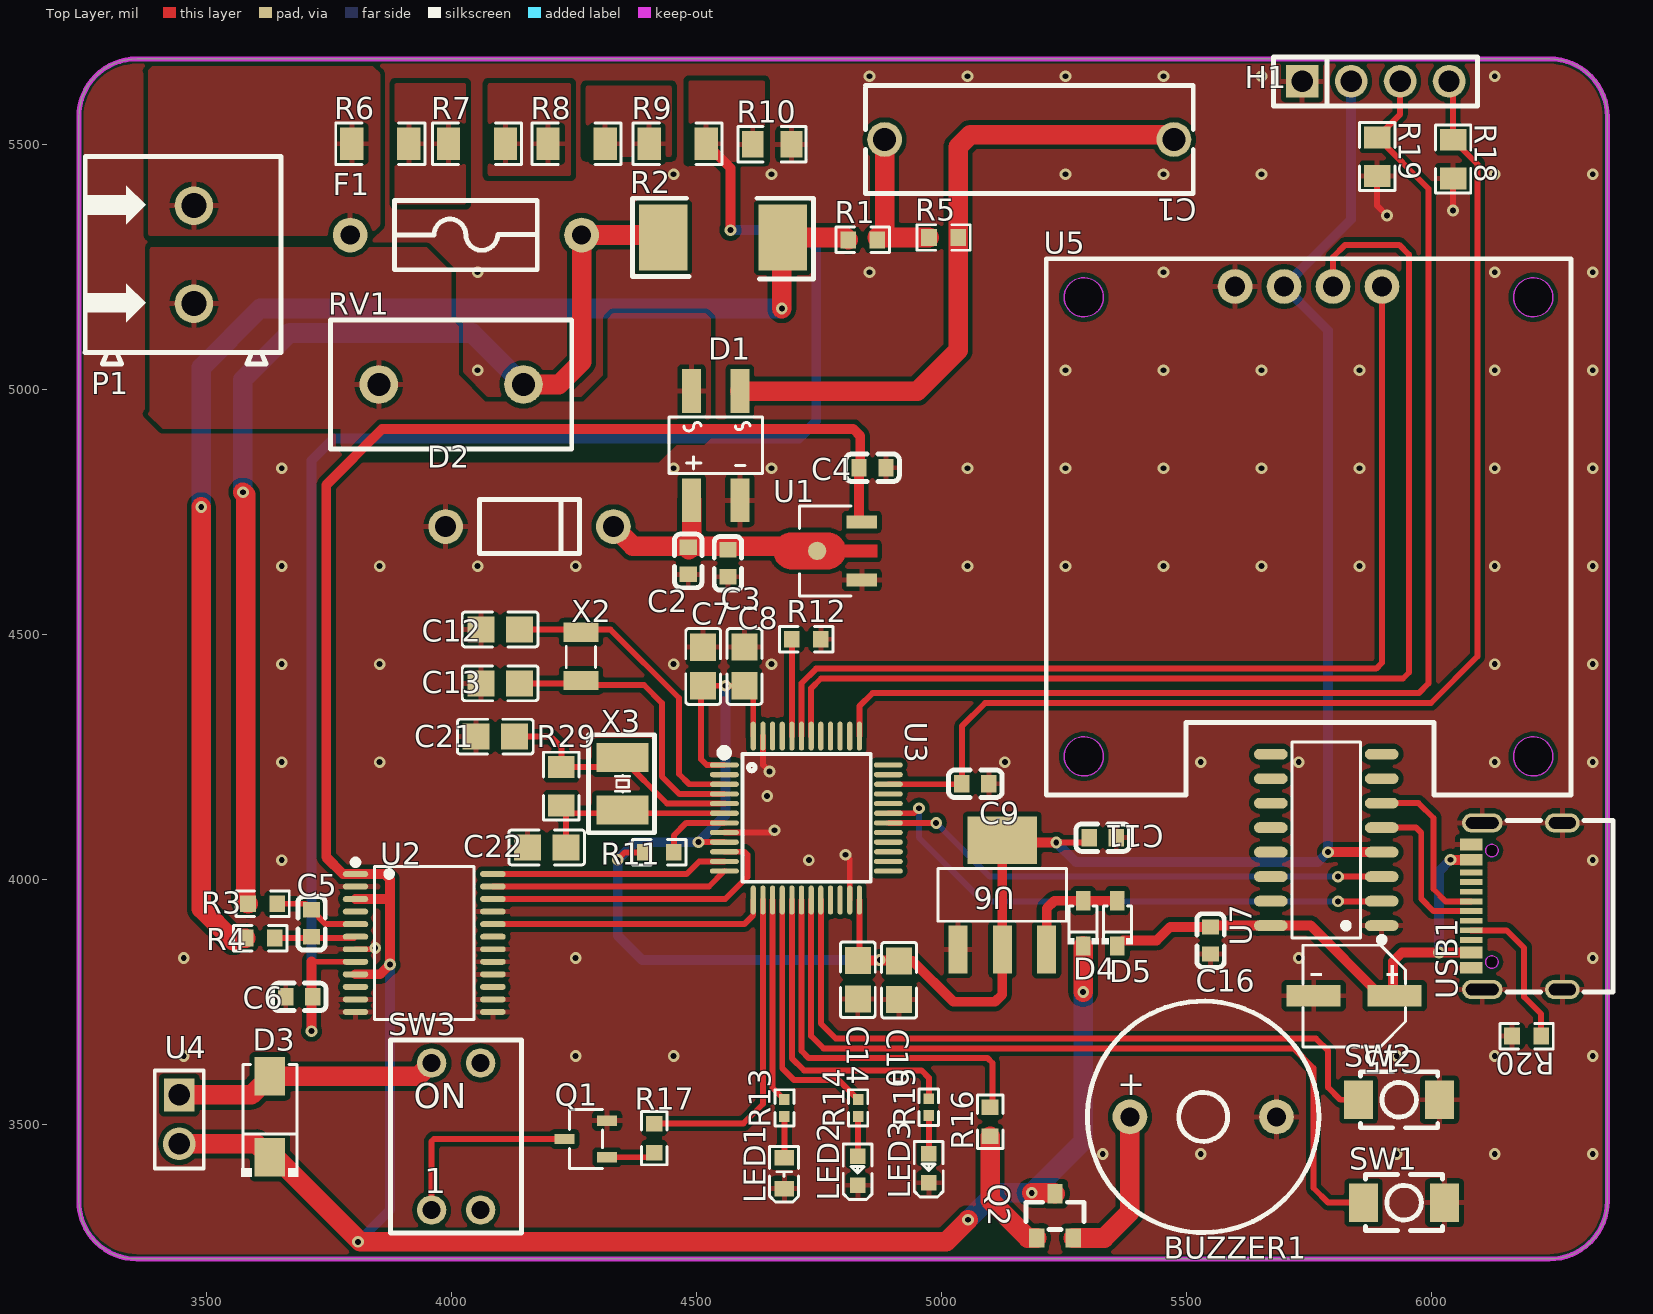
[diagram p0: Top Layer view]
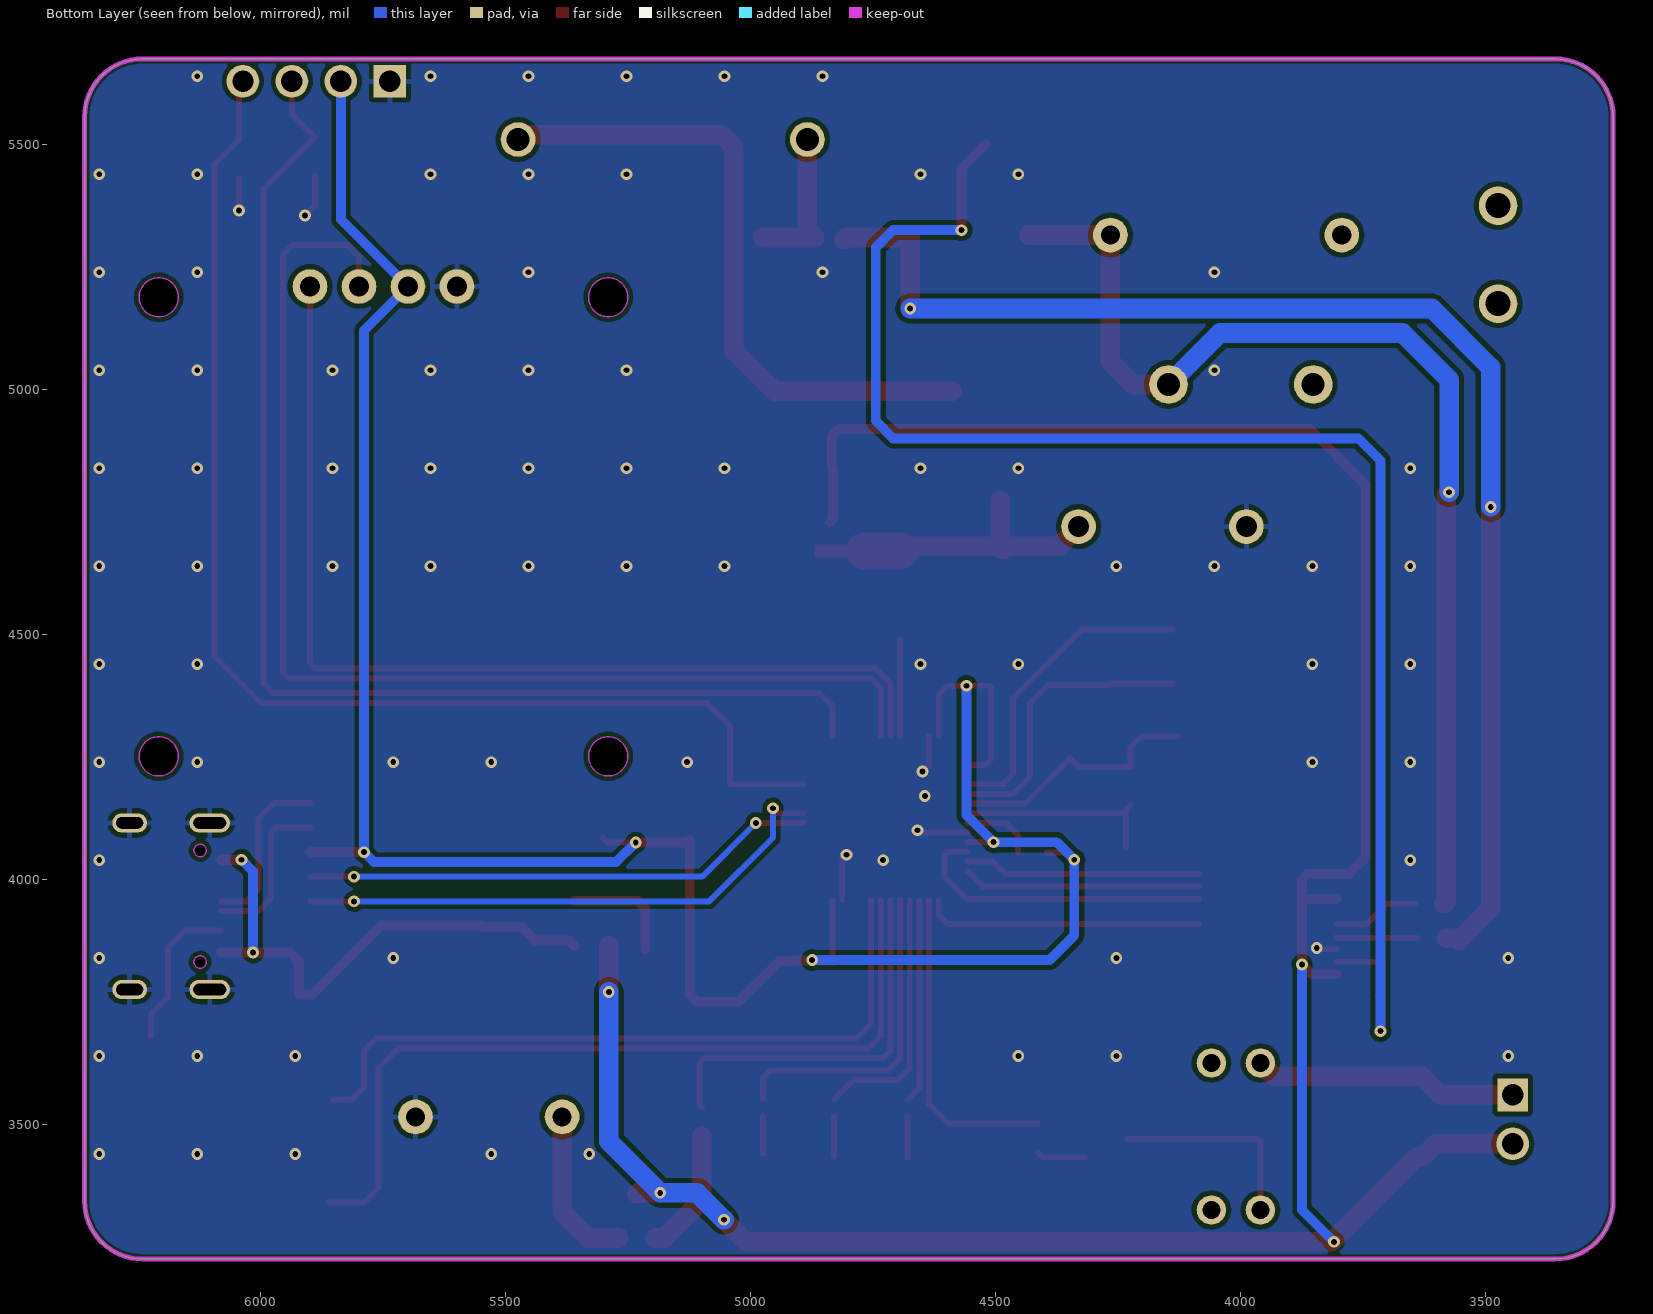
[diagram p1: Bottom Layer view, seen from below]
# Altium PCB MISC61242.pcbdoc
Units mil, origin at the board's own origin, x right, y up, seen from the top; angles counter-clockwise.
Board outline 3120 x 2449.61 mil, 2 copper layers (Top Layer, Bottom Layer), stack 2.757 mil thick; 67 components, 52 nets, 243 pads, 106 vias.

## Layer stack, top to bottom
Top Solder Mask Layer: solder mask 0.394, Dk 3.3
Top Layer: signal copper 1.379
Bottom Layer: signal copper 1.378
Bottom Solder Mask Layer: solder mask 0.394, Dk 3.3

## Board outline
3358.11,5674.61 ccw(c3358.11,5556.5) 3240,5556.5 3240,3343.11 ccw(c3358.11,3343.11) 3358.11,3225 6241.89,3225 ccw(c6241.89,3343.11) 6360,3343.11 6360,5556.5 ccw(c6241.89,5556.5) 6241.89,5674.61 3358.11,5674.61

## Design rules (kind name [scope] priority, off if disabled: settings)
BoardOutlineClearance Plane_innerPlane_1 [All] p2 off: genericclearance=4 ignorepadtopadclearanceinfootprint=FALSE except(0: Arc-SplitContinuation Track-SplitContinuation SMDPad-SplitContinuation THPad-SplitContinuation Via-SplitContinuation Fill-SplitContinuation Region-SplitContinuation Poly-SplitContinuation Text-SplitContinuation Hole-SplitContinuation; 6: Arc-CutoutEdge Track-CutoutEdge SMDPad-CutoutEdge THPad-CutoutEdge Via-CutoutEdge Text-CutoutEdge; 6.9: Hole-OutlineEdge Hole-CutoutEdge; 10: Poly-OutlineEdge Poly-CutoutEdge; 11.8: Arc-OutlineEdge Track-OutlineEdge SMDPad-OutlineEdge THPad-OutlineEdge Via-OutlineEdge Fill-OutlineEdge Region-OutlineEdge Text-OutlineEdge Fill-CutoutEdge Region-CutoutEdge)
BoardOutlineClearance Copper_copperRegion_1 [All] p4 off: genericclearance=4 ignorepadtopadclearanceinfootprint=FALSE except(0: Arc-SplitContinuation Track-SplitContinuation SMDPad-SplitContinuation THPad-SplitContinuation Via-SplitContinuation Fill-SplitContinuation Region-SplitContinuation Poly-SplitContinuation Text-SplitContinuation Hole-SplitContinuation; 6: Arc-CutoutEdge Track-CutoutEdge SMDPad-CutoutEdge THPad-CutoutEdge Via-CutoutEdge Text-CutoutEdge; 6.9: Hole-OutlineEdge Hole-CutoutEdge; 10: Poly-OutlineEdge Poly-CutoutEdge; 11.8: Arc-OutlineEdge Track-OutlineEdge SMDPad-OutlineEdge THPad-OutlineEdge Via-OutlineEdge Fill-OutlineEdge Region-OutlineEdge Text-OutlineEdge Fill-CutoutEdge Region-CutoutEdge)
BoardOutlineClearance Copper_copperRegion_copperThickness1oz_1 [All] p6 off: genericclearance=4 ignorepadtopadclearanceinfootprint=FALSE except(0: Arc-SplitContinuation Track-SplitContinuation SMDPad-SplitContinuation THPad-SplitContinuation Via-SplitContinuation Fill-SplitContinuation Region-SplitContinuation Poly-SplitContinuation Text-SplitContinuation Hole-SplitContinuation; 6: Arc-CutoutEdge Track-CutoutEdge SMDPad-CutoutEdge THPad-CutoutEdge Via-CutoutEdge Text-CutoutEdge; 6.9: Hole-OutlineEdge Hole-CutoutEdge; 10: Poly-OutlineEdge Poly-CutoutEdge; 11.8: Arc-OutlineEdge Track-OutlineEdge SMDPad-OutlineEdge THPad-OutlineEdge Via-OutlineEdge Fill-OutlineEdge Region-OutlineEdge Text-OutlineEdge Fill-CutoutEdge Region-CutoutEdge)
BoardOutlineClearance Copper_copperRegion_Copper_copperRegion_1 [All] p8 off: genericclearance=4 ignorepadtopadclearanceinfootprint=FALSE except(0: Arc-SplitContinuation Track-SplitContinuation SMDPad-SplitContinuation THPad-SplitContinuation Via-SplitContinuation Fill-SplitContinuation Region-SplitContinuation Poly-SplitContinuation Text-SplitContinuation Hole-SplitContinuation; 6: Arc-CutoutEdge Track-CutoutEdge SMDPad-CutoutEdge THPad-CutoutEdge Via-CutoutEdge Text-CutoutEdge; 6.9: Hole-OutlineEdge Hole-CutoutEdge; 10: Poly-OutlineEdge Poly-CutoutEdge; 11.8: Arc-OutlineEdge Track-OutlineEdge SMDPad-OutlineEdge THPad-OutlineEdge Via-OutlineEdge Fill-OutlineEdge Region-OutlineEdge Text-OutlineEdge Fill-CutoutEdge Region-CutoutEdge)
BoardOutlineClearance copperThickness1oz_1 [All] p10: genericclearance=4 ignorepadtopadclearanceinfootprint=FALSE except(0: Arc-SplitContinuation Track-SplitContinuation SMDPad-SplitContinuation THPad-SplitContinuation Via-SplitContinuation Fill-SplitContinuation Region-SplitContinuation Poly-SplitContinuation Text-SplitContinuation Hole-SplitContinuation; 6: Arc-CutoutEdge Track-CutoutEdge SMDPad-CutoutEdge THPad-CutoutEdge Via-CutoutEdge Text-CutoutEdge; 6.9: Hole-OutlineEdge Hole-CutoutEdge; 10: Poly-OutlineEdge Poly-CutoutEdge; 11.8: Arc-OutlineEdge Track-OutlineEdge SMDPad-OutlineEdge THPad-OutlineEdge Via-OutlineEdge Fill-OutlineEdge Region-OutlineEdge Text-OutlineEdge Fill-CutoutEdge Region-CutoutEdge)
Clearance Plane_innerPlane [All] p1 off: gap=4 ignorepadtopadclearanceinfootprint=FALSE except(6: SMDPad-Track SMDPad-SMDPad THPad-Track SMDPad-THPad THPad-THPad Track-Via SMDPad-Via THPad-Via Via-Via Fill-SMDPad Region-SMDPad Fill-THPad Region-THPad Fill-Via Region-Via Fill-Fill Fill-Region Region-Region Arc-Track Arc-SMDPad Arc-THPad Arc-Via Fill-Arc Region-Arc Arc-Arc Text-Track SMDPad-Text Text-THPad Text-Via Fill-Text Region-Text Arc-Text Text-Text; 6.9: Hole-Track Hole-SMDPad Hole-THPad Hole-Via Fill-Hole Region-Hole Hole-Arc Hole-Text; 10: Poly-Track Poly-SMDPad Poly-THPad Poly-Via Poly-Fill Poly-Region Poly-Poly Poly-Arc Poly-Text Poly-Hole; 11.8: Fill-Track Region-Track)
Clearance Copper_copperRegion [All] p3 off: gap=4 ignorepadtopadclearanceinfootprint=FALSE except(6: SMDPad-Track SMDPad-SMDPad THPad-Track SMDPad-THPad THPad-THPad Track-Via SMDPad-Via THPad-Via Via-Via Fill-SMDPad Region-SMDPad Fill-THPad Region-THPad Fill-Via Region-Via Fill-Fill Fill-Region Region-Region Arc-Track Arc-SMDPad Arc-THPad Arc-Via Fill-Arc Region-Arc Arc-Arc Text-Track SMDPad-Text Text-THPad Text-Via Fill-Text Region-Text Arc-Text Text-Text; 6.9: Hole-Track Hole-SMDPad Hole-THPad Hole-Via Fill-Hole Region-Hole Hole-Arc Hole-Text; 10: Poly-Track Poly-SMDPad Poly-THPad Poly-Via Poly-Fill Poly-Region Poly-Poly Poly-Arc Poly-Text Poly-Hole; 11.8: Fill-Track Region-Track)
Clearance Copper_copperRegion_copperThickness1oz [All] p5 off: gap=4 ignorepadtopadclearanceinfootprint=FALSE except(6: SMDPad-Track SMDPad-SMDPad THPad-Track SMDPad-THPad THPad-THPad Track-Via SMDPad-Via THPad-Via Via-Via Fill-SMDPad Region-SMDPad Fill-THPad Region-THPad Fill-Via Region-Via Fill-Fill Fill-Region Region-Region Arc-Track Arc-SMDPad Arc-THPad Arc-Via Fill-Arc Region-Arc Arc-Arc Text-Track SMDPad-Text Text-THPad Text-Via Fill-Text Region-Text Arc-Text Text-Text; 6.9: Hole-Track Hole-SMDPad Hole-THPad Hole-Via Fill-Hole Region-Hole Hole-Arc Hole-Text; 10: Poly-Track Poly-SMDPad Poly-THPad Poly-Via Poly-Fill Poly-Region Poly-Poly Poly-Arc Poly-Text Poly-Hole; 11.8: Fill-Track Region-Track)
Clearance Copper_copperRegion_Copper_copperRegion [All] p7 off: gap=4 ignorepadtopadclearanceinfootprint=FALSE except(6: SMDPad-Track SMDPad-SMDPad THPad-Track SMDPad-THPad THPad-THPad Track-Via SMDPad-Via THPad-Via Via-Via Fill-SMDPad Region-SMDPad Fill-THPad Region-THPad Fill-Via Region-Via Fill-Fill Fill-Region Region-Region Arc-Track Arc-SMDPad Arc-THPad Arc-Via Fill-Arc Region-Arc Arc-Arc Text-Track SMDPad-Text Text-THPad Text-Via Fill-Text Region-Text Arc-Text Text-Text; 6.9: Hole-Track Hole-SMDPad Hole-THPad Hole-Via Fill-Hole Region-Hole Hole-Arc Hole-Text; 10: Poly-Track Poly-SMDPad Poly-THPad Poly-Via Poly-Fill Poly-Region Poly-Poly Poly-Arc Poly-Text Poly-Hole; 11.8: Fill-Track Region-Track)
Clearance copperThickness1oz [All] p9: gap=4 ignorepadtopadclearanceinfootprint=FALSE except(6: SMDPad-Track SMDPad-SMDPad THPad-Track SMDPad-THPad THPad-THPad Track-Via SMDPad-Via THPad-Via Via-Via Fill-SMDPad Region-SMDPad Fill-THPad Region-THPad Fill-Via Region-Via Fill-Fill Fill-Region Region-Region Arc-Track Arc-SMDPad Arc-THPad Arc-Via Fill-Arc Region-Arc Arc-Arc Text-Track SMDPad-Text Text-THPad Text-Via Fill-Text Region-Text Arc-Text Text-Text; 6.9: Hole-Track Hole-SMDPad Hole-THPad Hole-Via Fill-Hole Region-Hole Hole-Arc Hole-Text; 10: Poly-Track Poly-SMDPad Poly-THPad Poly-Via Poly-Fill Poly-Region Poly-Poly Poly-Arc Poly-Text Poly-Hole; 11.8: Fill-Track Region-Track)
DiffPairsRouting differentialPair [All] p1: maxlimit=6 minlimit=5 mostfreqgap=6 toplayer_minwidth=5 toplayer_prefwidth=100 toplayer_maxwidth=100 toplayer_mingap=5 toplayer_prefgap=6 toplayer_maxgap=6 bottomlayer_minwidth=5 bottomlayer_prefwidth=100 bottomlayer_maxwidth=100 bottomlayer_mingap=5 bottomlayer_prefgap=6 bottomlayer_maxgap=6 maxuncoupledlength=10
HoleToHoleClearance otherClearance [All] p1: gap=11.8 allowstackedmicrovias=TRUE
Length netLength [All] p1: minlimit=0 maxlimit=0
PasteMaskExpansion pasteMaskExpansion [All] p1: expansion=0
PlaneConnect innerPlane [All] p1: planeconnectstyle=Relief reliefexpansion=20 reliefentries=4 reliefconductorwidth=10 reliefairgap=10
PolygonConnect copperRegion_copperThickness1oz [All] p1 off: connectstyle=Relief reliefconductorwidth=10 reliefentries=4 polygonreliefangle="90 Angle" airgapwidth=10 via.connectstyle=Relief via.reliefconductorwidth=10 via.reliefentries=4 via.polygonreliefangle="90 Angle" via.airgapwidth=10
PolygonConnect copperRegion_Copper_copperRegion [All] p2 off: connectstyle=Relief reliefconductorwidth=10 reliefentries=4 polygonreliefangle="90 Angle" airgapwidth=10 via.connectstyle=Relief via.reliefconductorwidth=10 via.reliefentries=4 via.polygonreliefangle="90 Angle" via.airgapwidth=10
PolygonConnect copperRegion [All] p3: connectstyle=Direct reliefconductorwidth=10 reliefentries=4 polygonreliefangle="90 Angle" airgapwidth=10 via.connectstyle=Relief via.reliefconductorwidth=10 via.reliefentries=4 via.polygonreliefangle="90 Angle" via.airgapwidth=10
RoutingVias viaSize [All] p1: holewidth=12 width=24 viastyle="Through Hole" minholewidth=1 minwidth=1 maxholewidth=393.7 maxwidth=248
SolderMaskExpansion solderMaskExpansion [IsVia] p1: expansion=-1000 istentingtop=TRUE
SolderMaskExpansion solderMaskExpansion [All] p2: expansion=2 istentingtop=FALSE
Width copperThickness1oz_2 [All] p1: maxlimit=100 minlimit=5 preferedwidth=10

## Components (designator, comment, footprint, x,y, rotation, side; value= is the part's Value field where it differs from the comment)
BUZZER1 "2.4kHz" BUZ-TH_BD12.0-P7.60-D0.6-FD 5535,3515 r0 top
C1 "470nF" CAP-TH_L17.0-W5.5-P15.00-D1.2 5180,5510 r180 top
C2 "47uF" C0603 4484.01,4649.76 r270 top
C3 "0.1μF" C0603 4565,4645 r270 top
C4 "10μF" C0603 4860,4840 r180 top
C5 "1nF" C0603 3715,3910 r90 top
C6 "1nF" C0603 3690,3760 r0 top
C7 "100nF" C0805 4514.37,4434.37 r90 top
C8 "100nF" C0805 4598.8,4434.51 r270 top
C9 "100nF" C0603 5070,4195 r180 top
C10 "100nF" C0805 4914.37,3793.97 r270 top
C11 "100nF" C0603 5330,4085 r180 top
C12 "20pF" C0805 4100,4510 r180 top
C13 "20pF" C0805 4100,4400 r0 top
C14 "100nF" C0805 4830,3795 r90 top
C15 "10uF" CAP-SMD_BD5.0-L5.3-W5.3-FD 5843.3,3762.26 r180 top
C16 "100nF" C0603 5550,3875 r90 top
C21 "20pF" C0805 4090.21,4291.12 r0 top
C22 "20pF" C0805 4195,4065 r0 top
D1 "MB10S" MBS_L4.7-W4.0-P2.50-LS7.0-TL 4540,4885 r270 top
D2 "1N4742" DO-41_BD2.4-L4.7-P8.70-D0.8-FD 4160,4720 r0 top
D3 "1N4007" SMA_L4.3-W2.5-LS5.0-RD 3630,3515 r90 top
D4 "1N5819WS" SOD-323_L1.8-W1.3-LS2.5-RD 5290,3910 r90 top
D5 "1N5819WS" SOD-323_L1.8-W1.3-LS2.5-RD 5360,3910 r90 top
F1 "2F.0500212000S1B02" FUSE-TH_BD3.0-L7.2-P11.20-D0.6 4030,5315 r0 top
H1 "" HDR-TH_4P-P2.54-V-F 5887,5628.78 r0 top
LED1 "NCD0603G1" LED0603-RD_1 4679.87,3400.05 r90 top
LED2 "NCD0603R1" LED0603-RD_RED 4830,3405 r90 top
LED3 "NCD0603Y1" LED0603-RD 4975,3410 r90 top
P1 "WJ500V-5.08-2P" CONN-TH_2P-P5.00_WJ500V-5.08-2P 3475,5275 r90 top
Q1 "S8050 J3Y(RANGE:200-350)" SOT-23-3_L3.0-W1.7-P0.95-LS2.9-BR 4275,3470 r0 top
Q2 "" S8050_SOT-23 5232.54,3313.14 r270 top
R1 "10Ω" R0603 4840,5305 r0 top
R2 "2mΩ" RES-SMD_L6.4-W3.2-1 4555,5310 r0 top
R3 "1K" R0603 3615,3950 r0 top
R4 "1K" R0603 3610,3880 r0 top
R5 "1MΩ" R0603 5005,5310 r0 top
R6 "1MΩ" R1206 3855.45,5501.36 r0 top
R7 "1MΩ" R1206 4052.86,5501.36 r0 top
R8 "1MΩ" R1206 4256.06,5501.36 r0 top
R9 "1MΩ" R1206 4462.27,5501.36 r0 top
R10 "10kΩ" R0805 4655,5500 r0 top
R11 "10K" R0603 4425,4055 r0 top
R12 "10K" R0603 4725,4490 r0 top
R13 "220Ω" R0402 4680.3,3533.26 r90 top
R14 "220Ω" R0402 4830.69,3533.26 r90 top
R15 "220Ω" R0402 4975,3535 r90 top
R16 "1KΩ" R0603 5100,3505 r90 top
R17 "1KΩ" R0603 4414.48,3471.81 r270 top
R18 "10kΩ" R0805 6045,5470 r270 top
R19 "10kΩ" R0805 5890,5475 r270 top
R20 "5.1K" R0603 6195,3680 r180 top
R29 "1M" R0805 4225,4190 r90 top
RV1 "190pF@1kHz" RES-TH_L12.5-W6.7-P7.50-D1.2 4000,5010 r0 top
SW1 "TS3425A2P 250gf" SW-SMD_L3.9-W2.9-LS5.0 5945,3340 r0 top
SW2 "TS3425A2P 250gf" SW-SMD_L3.9-W2.9-LS5.0 5935,3550 r0 top
SW3 "BSE02GR" SW-TH_4P-L9.9-W6.8-P7.62-BL 4010,3475 r0 top
U1 "HT7550-1" SOT-89_L4.5-W2.5-P1.50-LS4.2-BR 4785,4670 r0 top
U2 "ADE7755ARSZ" SSOP-24_L8.1-W5.3-P0.65-LS7.8-BL 3945,3870 r270 top
U3 "STM32F030C8T6TR" LQFP-48_L7.0-W7.0-P0.50-LS9.0-BL 4725,4125 r270 top
U4 "KF301-5.0-2P" HDR-M-2.54_1X2 3445,3510 r270 top
U5 "HS96L03W2C03" OLED-TH_L27.8-W27.2-P2.54_C9900033791 5750,5210 r0 top
U6 "AMS1117-3.3" SOT-223-4_L6.5-W3.5-P2.30-LS7.0-BR 5125,3968.34 r270 top
U7 "CH340C" SOP-16_L10.0-W3.9-P1.27-LS6.0-BL 5786.23,4080.41 r90 top
USB1 "TYPE-C16PIN" USB-C-SMD_TYPE-C16PIN 6175,3945 r90 top
X2 "32.768kHz" CRYSTAL-SMD_L3.2-W1.5-FC-135R32.7680KF-A3 4265,4455 r270 top
X3 "8MHz" CRYSTAL-SMD_L3.2-W2.5_3225-8MHZ 4350,4195 r90 top

## Footprints (in the part's own frame and the unit in brackets; to place one, negate y for a bottom-side part, rotate by r counter-clockwise, add the part's x,y. Pads: shape width x height; smd on the part's side, far side on the other; paste and mask are expansions set on the pad)
BUZ-TH_BD12.0-P7.60-D0.6-FD [mm]
  round 1.8 hole 1: 1(-3.8,0) 2(3.8,0)
  silkscreen extent -6,-6 6,6
C0603 [mm]
  rect 0.8x0.9 smd: 1(-0.7,0) 2(0.7,0)
  silkscreen extent -1.39,-0.71 1.39,0.71
C0805 [mm]
  rect 1.41x1.35 smd paste-100 mask+0.051: 1(-1,0) 2(1,0)
  silkscreen extent -1.96,-0.9 1.96,0.9
CAP-SMD_BD5.0-L5.3-W5.3-FD [mm]
  rect 2.8x1.1 smd: 1(-2.1,0) 2(2.1,0)
  silkscreen extent -2.66,-2.62 2.66,2.65
CAP-TH_L17.0-W5.5-P15.00-D1.2 [mm]
  round 1.8 hole 1.2: 1(-7.501,0) 2(7.501,0)
  silkscreen extent -8.5,-2.8 8.5,2.8
CONN-TH_2P-P5.00_WJ500V-5.08-2P [mm]
  round 2 hole 1.3: 1(-2.54,0) 2(2.54,0)
  silkscreen extent -5.68,-4.52 5.08,5.64
CRYSTAL-SMD_L3.2-W1.5-FC-135R32.7680KF-A3 [mm]
  rect 1x1.8 smd paste+0 mask+0.05: 1(-1.25,0) 2(1.25,0)
  silkscreen extent -0.51,-0.76 0.57,0.76
CRYSTAL-SMD_L3.2-W2.5_3225-8MHZ [mil]
  rect 60x106.3 smd paste+0 mask+1.97: 1(-53.62,0) 2(53.62,0)
  silkscreen extent -100,-65 100,70
DO-41_BD2.4-L4.7-P8.70-D0.8-FD [mm]
  round 1.8 hole 1.1: 1(-4.35,0) 2(4.35,0)
  silkscreen extent -2.6,-1.4 2.6,1.4
FUSE-TH_BD3.0-L7.2-P11.20-D0.6 [mm]
  round 1.8 hole 1: 1(-6,0) 2(6,0)
  silkscreen extent -3.7,-1.8 3.7,1.8
HDR-M-2.54_1X2 [mm]
  rect 1.7x1.575 hole 1.1: 1(-1.27,0)
  round 1.7 hole 1.1: 2(1.27,0)
  silkscreen extent -2.54,-1.27 2.54,1.27
HDR-TH_4P-P2.54-V-F [mm]
  rect 1.7x1.7 hole 1.1: 1(-3.81,0)
  round 1.7 hole 1.1: 2(-1.27,0) 3(1.27,0) 4(3.81,0)
  silkscreen extent -5.29,-1.27 5.29,1.27
LED0603-RD [mm]
  rect 0.8x0.8 smd: 1(-0.749,0) 2(0.749,0)
  silkscreen extent -1.49,-0.75 1.39,0.76
LED0603-RD_1 [mm]
  rect 0.8x1 smd: 1(-0.799,-0.004) 2(0.799,0.004)
  silkscreen extent -1.49,-0.75 1.39,0.76
LED0603-RD_RED [mm]
  rect 0.8x0.8 smd: 1(-0.749,-0.003) 2(0.749,0.003)
  silkscreen extent -1.49,-0.75 1.39,0.76
LQFP-48_L7.0-W7.0-P0.50-LS9.0-BL [mm]
  oval 0.27x1.5 smd paste+0 mask+0.05: 1(-2.75,-4.25) 2(-2.25,-4.25) 3(-1.75,-4.25) 4(-1.25,-4.25) 5(-0.75,-4.25) 6(-0.25,-4.25) 7(0.25,-4.25) 8(0.75,-4.25) 9(1.25,-4.25) 10(1.75,-4.25) 11(2.25,-4.25) 12(2.75,-4.25) 25(2.75,4.25) 26(2.25,4.25) 27(1.75,4.25) 28(1.25,4.25) 29(0.75,4.25) 30(0.25,4.25) 31(-0.25,4.25) 32(-0.75,4.25) 33(-1.25,4.25) 34(-1.75,4.25) 35(-2.25,4.25) 36(-2.75,4.25)
  oval 1.5x0.27 smd paste+0 mask+0.05: 13(4.25,-2.75) 14(4.25,-2.25) 15(4.25,-1.75) 16(4.25,-1.25) 17(4.25,-0.75) 18(4.25,-0.25) 19(4.25,0.25) 20(4.25,0.75) 21(4.25,1.25) 22(4.25,1.75) 23(4.25,2.25) 24(4.25,2.75) 37(-4.25,2.75) 38(-4.25,2.25) 39(-4.25,1.75) 40(-4.25,1.25) 41(-4.25,0.75) 42(-4.25,0.25) 43(-4.25,-0.25) 44(-4.25,-0.75) 45(-4.25,-1.25) 46(-4.25,-1.75) 47(-4.25,-2.25) 48(-4.25,-2.75)
  silkscreen extent -3.59,-4.46 3.3,3.34
MBS_L4.7-W4.0-P2.50-LS7.0-TL [mm]
  rect 2.265x0.98 smd: 1(-2.832,1.25) 2(-2.832,-1.25) 3(2.832,-1.25) 4(2.832,1.25)
  silkscreen extent -1.5,-2.43 1.44,2.43
OLED-TH_L27.8-W27.2-P2.54_C9900033791 [mm]
  round 1.8 hole 1.05 paste+0 mask+0.05: 1(-3.81,0) 2(-1.27,0) 3(1.27,0) 4(3.81,0)
  Board Outline Layer circle w0.003: c-11.65,-0.56 r1.016
  Board Outline Layer circle w0.003: c11.65,-0.56 r1.016
  Board Outline Layer circle w0.003: c-11.65,-24.36 r1.016
  Board Outline Layer circle w0.003: c11.65,-24.36 r1.016
  Board Outline Layer region: -10.634,-0.56 -10.735,-1.001 -11.016,-1.354 -11.424,-1.551 -11.876,-1.551 -12.283,-1.354 -12.565,-1.001 -12.666,-0.56 -12.666,-0.56 -12.565,-0.119 -12.283,0.234 -11.876,0.431 -11.424,0.431 -11.016,0.234 -10.735,-0.119 -10.634,-0.56
  Board Outline Layer region: -10.634,-0.56 -10.643,-0.698 -10.672,-0.834 -10.718,-0.965 -10.782,-1.088 -10.862,-1.201 -10.956,-1.303 -11.064,-1.39 -11.183,-1.462 -11.31,-1.517 -11.443,-1.555 -11.581,-1.574 -11.719,-1.574 -11.857,-1.555 -11.99,-1.517 -12.117,-1.462 -12.236,-1.39 -12.343,-1.303 -12.438,-1.201 -12.518,-1.088 -12.582,-0.965 -12.628,-0.834 -12.656,-0.698 -12.666,-0.56 -12.656,-0.422 -12.628,-0.286 -12.582,-0.155 -12.518,-0.032 -12.438,0.081 -12.343,0.183 -12.236,0.27 -12.117,0.342 -11.99,0.397 -11.857,0.435 -11.719,0.454 -11.581,0.454 -11.443,0.435 -11.31,0.397 -11.183,0.342 -11.064,0.27 -10.956,0.183 -10.862,0.081 -10.782,-0.032 -10.718,-0.155 -10.672,-0.286 -10.643,-0.422
  Board Outline Layer region: 12.666,-0.56 12.565,-1.001 12.283,-1.354 11.876,-1.551 11.424,-1.551 11.017,-1.354 10.735,-1.001 10.634,-0.56 10.634,-0.56 10.735,-0.119 11.017,0.234 11.424,0.431 11.876,0.431 12.283,0.234 12.565,-0.119 12.666,-0.56
  Board Outline Layer region: 12.666,-0.56 12.657,-0.698 12.628,-0.834 12.582,-0.965 12.518,-1.088 12.438,-1.201 12.343,-1.303 12.236,-1.39 12.117,-1.462 11.99,-1.517 11.857,-1.555 11.719,-1.574 11.581,-1.574 11.443,-1.555 11.31,-1.517 11.183,-1.462 11.064,-1.39 10.957,-1.303 10.862,-1.201 10.782,-1.088 10.718,-0.965 10.672,-0.834 10.643,-0.698 10.634,-0.56 10.643,-0.422 10.672,-0.286 10.718,-0.155 10.782,-0.032 10.862,0.081 10.957,0.183 11.064,0.27 11.183,0.342 11.31,0.397 11.443,0.435 11.581,0.454 11.719,0.454 11.857,0.435 11.99,0.397 12.117,0.342 12.236,0.27 12.343,0.183 12.438,0.081 12.518,-0.032 12.582,-0.155 12.628,-0.286 12.657,-0.422
  Board Outline Layer region: -10.634,-24.36 -10.735,-24.801 -11.016,-25.154 -11.424,-25.35 -11.876,-25.35 -12.283,-25.154 -12.565,-24.801 -12.666,-24.36 -12.666,-24.36 -12.565,-23.919 -12.283,-23.566 -11.876,-23.369 -11.424,-23.369 -11.016,-23.566 -10.735,-23.919 -10.634,-24.36
  Board Outline Layer region: -10.634,-24.36 -10.643,-24.498 -10.672,-24.634 -10.718,-24.765 -10.782,-24.888 -10.862,-25.001 -10.956,-25.102 -11.064,-25.19 -11.183,-25.262 -11.31,-25.317 -11.443,-25.355 -11.581,-25.374 -11.719,-25.374 -11.857,-25.355 -11.99,-25.317 -12.117,-25.262 -12.236,-25.19 -12.343,-25.102 -12.438,-25.001 -12.518,-24.888 -12.582,-24.765 -12.628,-24.634 -12.656,-24.498 -12.666,-24.36 -12.656,-24.222 -12.628,-24.086 -12.582,-23.955 -12.518,-23.832 -12.438,-23.719 -12.343,-23.617 -12.236,-23.53 -12.117,-23.458 -11.99,-23.403 -11.857,-23.365 -11.719,-23.346 -11.581,-23.346 -11.443,-23.365 -11.31,-23.403 -11.183,-23.458 -11.064,-23.53 -10.956,-23.617 -10.862,-23.719 -10.782,-23.832 -10.718,-23.955 -10.672,-24.086 -10.643,-24.222
  Board Outline Layer region: 12.666,-24.36 12.565,-24.801 12.283,-25.154 11.876,-25.35 11.424,-25.35 11.017,-25.154 10.735,-24.801 10.634,-24.36 10.634,-24.36 10.735,-23.919 11.017,-23.566 11.424,-23.369 11.876,-23.369 12.283,-23.566 12.565,-23.919 12.666,-24.36
  Board Outline Layer region: 12.666,-24.36 12.657,-24.498 12.628,-24.634 12.582,-24.765 12.518,-24.888 12.438,-25.001 12.343,-25.102 12.236,-25.19 12.117,-25.262 11.99,-25.317 11.857,-25.355 11.719,-25.374 11.581,-25.374 11.443,-25.355 11.31,-25.317 11.183,-25.262 11.064,-25.19 10.957,-25.102 10.862,-25.001 10.782,-24.888 10.718,-24.765 10.672,-24.634 10.643,-24.498 10.634,-24.36 10.643,-24.222 10.672,-24.086 10.718,-23.955 10.782,-23.832 10.862,-23.719 10.957,-23.617 11.064,-23.53 11.183,-23.458 11.31,-23.403 11.443,-23.365 11.581,-23.346 11.719,-23.346 11.857,-23.365 11.99,-23.403 12.117,-23.458 12.236,-23.53 12.343,-23.617 12.438,-23.719 12.518,-23.832 12.582,-23.955 12.628,-24.086 12.657,-24.222
  Multi-Layer board cut-out: -10.634,-0.56 -10.735,-1.001 -11.016,-1.354 -11.424,-1.551 -11.876,-1.551 -12.283,-1.354 -12.565,-1.001 -12.666,-0.56 -12.666,-0.56 -12.565,-0.119 -12.283,0.234 -11.876,0.431 -11.424,0.431 -11.016,0.234 -10.735,-0.119 -10.634,-0.56
  Multi-Layer board cut-out: 12.666,-0.56 12.565,-1.001 12.283,-1.354 11.876,-1.551 11.424,-1.551 11.017,-1.354 10.735,-1.001 10.634,-0.56 10.634,-0.56 10.735,-0.119 11.017,0.234 11.424,0.431 11.876,0.431 12.283,0.234 12.565,-0.119 12.666,-0.56
  Multi-Layer board cut-out: -10.634,-24.36 -10.735,-24.801 -11.016,-25.154 -11.424,-25.35 -11.876,-25.35 -12.283,-25.154 -12.565,-24.801 -12.666,-24.36 -12.666,-24.36 -12.565,-23.919 -12.283,-23.566 -11.876,-23.369 -11.424,-23.369 -11.016,-23.566 -10.735,-23.919 -10.634,-24.36
  Multi-Layer board cut-out: 12.666,-24.36 12.565,-24.801 12.283,-25.154 11.876,-25.35 11.424,-25.35 11.017,-25.154 10.735,-24.801 10.634,-24.36 10.634,-24.36 10.735,-23.919 11.017,-23.566 11.424,-23.369 11.876,-23.369 12.283,-23.566 12.565,-23.919 12.666,-24.36
  silkscreen extent -13.6,-26.36 13.6,1.44
R0402 [mm]
  rect 0.566x0.54 smd paste-100 mask+0.051: 1(-0.433,0) 2(0.433,0)
  silkscreen extent -0.94,-0.5 0.94,0.5
R0603 [mil]
  rect 31.75x34.02 smd paste-3937.01 mask+2: 1(-29.66,0) 2(29.66,0)
  silkscreen extent -55,-26 55,26
R0805 [mm]
  rect 1.133x1.377 smd paste-100 mask+0.051: 1(-1,0) 2(1,0)
  silkscreen extent -1.76,-0.92 1.76,0.92
R1206 [mil]
  rect 47.54x66.97 smd paste-3937.01 mask+2: 1(-58.22,0) 2(58.22,0)
  silkscreen extent -91,-42 91,42
RES-SMD_L6.4-W3.2-1 [mm]
  rect 2.5x3.4 smd: 1(-3.1,0) 2(3.1,0)
  silkscreen extent -4.69,-2.16 4.69,2.03
RES-TH_L12.5-W6.7-P7.50-D1.2 [mm]
  round 2 hole 1.2: 1(-3.749,0) 2(3.749,0)
  silkscreen extent -6.25,-3.35 6.25,3.35
S8050_SOT-23 [mm]
  rect 1x0.8 smd paste+0 mask+0.051: 1(1.15,-0.95) 2(1.15,0.95) 3(-1.15,0)
  silkscreen extent -0.7,-1.5 0.7,1.5
SMA_L4.3-W2.5-LS5.0-RD [mm]
  rect 2x1.593 smd: 1(-2.1,0) 2(2.1,0)
  silkscreen extent -3.11,-1.48 2.73,1.48
SOD-323_L1.8-W1.3-LS2.5-RD [mm]
  rect 1x0.75 smd: 1(-1.173,0) 2(1.173,0)
  silkscreen extent -1.08,-0.8 0.9,0.8
SOP-16_L10.0-W3.9-P1.27-LS6.0-BL [mm]
  oval 0.56x1.745 smd: 1(-4.445,-2.872) 2(-3.175,-2.872) 3(-1.905,-2.872) 4(-0.635,-2.872) 5(0.635,-2.872) 6(1.905,-2.872) 7(3.175,-2.872) 8(4.445,-2.872) 9(4.445,2.872) 10(3.175,2.872) 11(1.905,2.872) 12(0.635,2.872) 13(-0.635,2.872) 14(-1.905,2.872) 15(-3.175,2.872) 16(-4.445,2.872)
  silkscreen extent -5.33,-3.02 5.08,1.77
SOT-23-3_L3.0-W1.7-P0.95-LS2.9-BR [mil]
  rect 40.85x20.95 smd: 1(43.36,-37.4) 2(43.36,37.4) 3(-43.36,0)
  silkscreen extent -34,-60 34,60
SOT-89_L4.5-W2.5-P1.50-LS4.2-BR [mm]
  rect 1.575x0.672 smd: 1(1.356,-1.5) 3(1.356,1.5)
  round 0.95 smd: 2(-0.966,0.009)
  Top Layer region: -2.283,0.959 -0.429,0.959 -0.385,0.958 -0.34,0.955 -0.296,0.949 -0.252,0.942 -0.208,0.933 -0.165,0.921 -0.123,0.908 -0.081,0.893 -0.04,0.875 0,0.856 0.04,0.835 0.078,0.812 0.115,0.788 0.151,0.761 0.185,0.733 0.219,0.704 0.251,0.673 0.281,0.64 0.31,0.606 0.337,0.571 0.362,0.534 0.386,0.497 0.408,0.458 0.428,0.418 0.447,0.339 2.144,0.339 2.144,-0.321 0.447,-0.321 0.428,-0.401 0.408,-0.44 0.386,-0.479 0.362,-0.517 0.337,-0.553 0.31,-0.588 0.281,-0.622 0.251,-0.655 0.219,-0.686 0.185,-0.716 0.151,-0.744 0.115,-0.77 0.078,-0.795 0.04,-0.818 0,-0.839 -0.04,-0.858 -0.081,-0.875 -0.123,-0.89 -0.165,-0.904 -0.208,-0.915 -0.252,-0.925 -0.296,-0.932 -0.34,-0.937 -0.385,-0.94 -0.429,-0.941 -2.283,-0.941 -2.328,-0.94 -2.372,-0.937 -2.416,-0.932 -2.46,-0.925 -2.504,-0.915 -2.547,-0.904 -2.589,-0.89 -2.631,-0.875 -2.672,-0.858 -2.713,-0.839 -2.752,-0.818 -2.79,-0.795 -2.827,-0.77 -2.863,-0.744 -2.898,-0.716 -2.931,-0.686 -2.963,-0.655 -2.993,-0.622 -3.022,-0.588 -3.049,-0.553 -3.075,-0.517 -3.098,-0.479 -3.12,-0.44 -3.141,-0.401 -3.159,-0.36 -3.175,-0.318 -3.189,-0.276 -3.202,-0.233 -3.212,-0.19 -3.22,-0.146 -3.227,-0.102 -3.231,-0.058 -3.233,-0.013 -3.233,0.031 -3.231,0.076 -3.227,0.12 -3.22,0.164 -3.212,0.208 -3.202,0.251 -3.189,0.294 -3.175,0.336 -3.159,0.377 -3.141,0.418 -3.12,0.458 -3.098,0.497 -3.075,0.534 -3.049,0.571 -3.022,0.606 -2.993,0.64 -2.963,0.673 -2.931,0.704 -2.898,0.733 -2.863,0.761 -2.827,0.788 -2.79,0.812 -2.752,0.835 -2.713,0.856 -2.672,0.875 -2.631,0.893 -2.589,0.908 -2.547,0.921 -2.504,0.933 -2.46,0.942 -2.416,0.949 -2.372,0.955 -2.328,0.958
  silkscreen extent -1.87,-2.33 0.78,2.33
SOT-223-4_L6.5-W3.5-P2.30-LS7.0-BR [mm]
  rect 2.47x0.98 smd: 1(2.835,-2.3) 2(2.835,0) 3(2.835,2.3)
  rect 2.47x3.6 smd: 4(-2.835,0)
  silkscreen extent -1.37,-3.33 1.37,3.33
SSOP-24_L8.1-W5.3-P0.65-LS7.8-BL [mil]
  oval 12.13x52.13 smd: 1(-140.75,-140.24) 2(-115.16,-140.24) 3(-89.57,-140.24) 4(-63.98,-140.24) 5(-38.39,-140.24) 6(-12.79,-140.24) 7(12.8,-140.24) 8(38.39,-140.24) 9(63.98,-140.24) 10(89.57,-140.24) 11(115.16,-140.24) 12(140.75,-140.24) 13(140.75,140.24) 14(115.16,140.24) 15(89.57,140.24) 16(63.98,140.24) 17(38.39,140.24) 18(12.8,140.24) 19(-12.79,140.24) 20(-38.39,140.24) 21(-63.98,140.24) 22(-89.57,140.24) 23(-115.16,140.24) 24(-140.75,140.24)
  silkscreen extent -171,-146 157,101
SW-SMD_L3.9-W2.9-LS5.0 [mm]
  rect 1.5x2 smd: 1(-2.1,0) 2(2.1,0)
  silkscreen extent -2,-1.45 2,1.45
SW-TH_4P-L9.9-W6.8-P7.62-BL [mil]
  round 60 hole 36 paste+0 mask+1.97: 1(-50,-150) 2(50,-150) 3(50,150) 4(-50,150)
  silkscreen extent -134,-197 134,197
USB-C-SMD_TYPE-C16PIN [mm]
  oval 1x2.1 hole 0.6 slot 1.7 at 90 deg: 1(-4.32,1.787) 2(4.32,1.787)
  oval 1x1.8 hole 0.6 slot 1.4 at 90 deg: 3(-4.32,-2.362) 4(4.32,-2.362)
  rect 0.6x1.15 smd paste-100 mask+0.051: A1B12(-3.2,2.362) A4B9(-2.4,2.362) B1A12(3.2,2.362) B4A9(2.4,2.362)
  rect 0.3x1.15 smd paste-100 mask+0.051: A5(-1.25,2.362) A6(-0.25,2.362) A7(0.25,2.362) A8(1.25,2.362) B5(1.75,2.362) B6(0.75,2.362) B7(-0.75,2.362) B8(-1.75,2.362)
  Board Outline Layer circle w0.003: c2.89,1.288 r0.325
  Board Outline Layer circle w0.003: c-2.89,1.288 r0.325
  Board Outline Layer region: 2.89,0.963 2.749,0.995 2.636,1.085 2.573,1.216 2.573,1.36 2.636,1.491 2.749,1.581 2.89,1.613 2.89,1.613 3.031,1.581 3.144,1.491 3.207,1.36 3.207,1.216 3.144,1.085 3.031,0.995 2.89,0.963
  Board Outline Layer region: 2.89,0.963 2.812,0.972 2.739,1 2.675,1.045 2.623,1.103 2.586,1.173 2.567,1.249 2.567,1.327 2.586,1.403 2.623,1.473 2.675,1.531 2.739,1.576 2.812,1.604 2.89,1.613 2.968,1.604 3.041,1.576 3.106,1.531 3.157,1.473 3.194,1.403 3.213,1.327 3.213,1.249 3.194,1.173 3.157,1.103 3.106,1.045 3.041,1 2.968,0.972
  Board Outline Layer region: -2.89,0.963 -3.031,0.995 -3.144,1.085 -3.207,1.216 -3.207,1.36 -3.144,1.491 -3.031,1.581 -2.89,1.613 -2.89,1.613 -2.749,1.581 -2.636,1.491 -2.573,1.36 -2.573,1.216 -2.636,1.085 -2.749,0.995 -2.89,0.963
  Board Outline Layer region: -2.89,0.963 -2.968,0.972 -3.041,1 -3.106,1.045 -3.157,1.103 -3.194,1.173 -3.213,1.249 -3.213,1.327 -3.194,1.403 -3.157,1.473 -3.106,1.531 -3.041,1.576 -2.968,1.604 -2.89,1.613 -2.812,1.604 -2.739,1.576 -2.675,1.531 -2.623,1.473 -2.586,1.403 -2.567,1.327 -2.567,1.249 -2.586,1.173 -2.623,1.103 -2.675,1.045 -2.739,1 -2.812,0.972
  Multi-Layer board cut-out: 2.89,0.963 2.749,0.995 2.636,1.085 2.573,1.216 2.573,1.36 2.636,1.491 2.749,1.581 2.89,1.613 2.89,1.613 3.031,1.581 3.144,1.491 3.207,1.36 3.207,1.216 3.144,1.085 3.031,0.995 2.89,0.963
  Multi-Layer board cut-out: -2.89,0.963 -3.031,0.995 -3.144,1.085 -3.207,1.216 -3.207,1.36 -3.144,1.491 -3.031,1.581 -2.89,1.613 -2.89,1.613 -2.749,1.581 -2.636,1.491 -2.573,1.36 -2.573,1.216 -2.636,1.085 -2.749,0.995 -2.89,0.963
  silkscreen extent -4.45,-5 4.45,0.52

## Via types
v1: diameter 24, hole 12, Top Layer to Bottom Layer, 106 vias

## Nets (pads, with @x,y where several pads share a name; then routed paths per layer and width w, separated by ;. In a path a pad name is that pad's centre, name@x,y a point inside that pad or via, vN(x,y) a via of type N, cw(c..) or ccw(c..) an arc to the next point about the centre after c; other vN are vias at no path point)
$1N1: F1.1 P1.2 R6.1
$1N9: C1.2 R1.2 R5.1 | length 311.9
  Top Layer w40: C1.2 4884.7,5325.04 4869.66,5310 R5.1
$1N13: C1.1 D1.1 R5.2 | length 1350.2
  Top Layer w40: D1.1 4951.52,4996.52 5034.66,5079.66 R5.2 5034.66,5494.66 5060,5520 5465.3,5520 C1.1
$1N47: C2.1 C3.1 D1.3 D2.2 U1.2 | length 524.2
  Top Layer w40: D2.2 4371.26,4680 C2.1@4490.78,4680 ; C2.1@4485,4672.56 4490.78,4678.34 C2.1@4490.78,4680 ; D1.3 C2.1@4490.78,4680 ; U1.2@4731.6,4670.34 4721.94,4680 C2.1@4490.78,4680
$1N59: C5.2 R3.2 U2.5 | length 177.3
  Top Layer w12: R3.2 3702.56,3950 C5.2 3744.17,3908.39 U2.5
$1N60: C5.1 R4.2 U2.6 | length 166.3
  Top Layer w12: R4.2 3801.97,3880 U2.6
$1N67: R6.2 R7.1
$1N68: R7.2 R8.1
$1N69: R8.2 R9.1
$1N81: R11.2 U3.7 | length 148.2
  Top Layer w12: R11.2 4454.66,4089.66 4480.16,4115.16 U3.7
$1N82: R12.1 U3.44 | length 197.7
  Top Layer w12: R12.1 4695.47,4489.87 U3.44
$1N86: LED1.2 R13.1 | length 84.9
  Top Layer w12: LED1.2 4680.3,3432.09 R13.1
$1N87: LED2.2 R14.1 | length 82.1
  Top Layer w12: LED2.2 4830.69,3435.31 R14.1
$1N88: LED3.2 R15.1 | length 78.5
  Top Layer w12: LED3.2 R15.1
$1N95: Q1.1 R17.2 | length 100.1
  Top Layer w12: Q1.1 4404.93,3432.6 R17.2
$1N96: Q1.3 SW3.1 | length 413.7
  Top Layer w12: SW3.1 3960,3465 3965,3470 Q1.3
$1N98: D3.2 SW3.4 U4.1 | length 541.9
  Top Layer w40: U4.1 3592.32,3560 D3.2 3932.68,3597.68 SW3.4
$1N109: D1.2 P1.1 RV1.1
$1N205: D4.2 D5.2 U6.3 | length 234.7
  Top Layer w20: U6.3 5215.55,3940.55 5231.16,3956.16 D4.2 D5.2
$1N215: R20.1 USB1.A5 | length 317.2
  Top Layer w12: USB1.A5 6154.21,3895.79 6190,3860 6190,3760 6224.66,3725.34 R20.1
$1N217: U7.5 USB1.A6 | length 332.3
  Top Layer w12: U7.5 5969.59,4105.41 5980,4095 5980,3960 6004.84,3935.16 USB1.A6
$1N218: U7.6 USB1.A7 | length 350.7
  Top Layer w12: U7.6 5974.59,4155.41 6005,4125 6005,3980 6030.16,3954.84 USB1.A7
$1N224: Q2.1 R16.1 | length 257.4
  Top Layer w40: R16.1 5100,3345 5177.14,3267.86 Q2.1
$1N225: BUZZER1.1 Q2.2 | length 331.8
  Top Layer w40: Q2.2 5332.86,3267.86 5385.4,3320.39 BUZZER1.1
$1N227: C15.1 C16.2 D5.1 U7.16 USB1.A4B9 USB1.B4A9 | length 1113.8
  Top Layer w20: D5.1 5371.16,3875 5440,3875 5467.56,3902.56 C16.2 5552.85,3905.41 U7.16 5754.59,3905.41 5895,3765 5922.32,3765 5922.32,3832.32 5940.51,3850.51 v1(6016.05,3850.51) USB1.A4B9 ; v1(6040,4040) 6040.51,4039.49 USB1.B4A9
  Bottom Layer w20: v1(6016.05,3850.51) 6016.05,4016.05 v1(6040,4040)
+5V: C4.2 D3.1 D4.1 Q2.3 U1.3 U2.1 U2.3 U2.9 U4.2 | length 5607
  Top Layer w20: U2.9 3855.11,3806.02 v1(3875,3825.91) 3875,3958.72 ; U2.3 3874.15,3959.57 3875,3958.72 ; U1.3 4832.44,4735.02 C4.2 4835,4842.56 4835,4905 4820.86,4919.14 3859.14,4919.14 3745,4805 3745,4045 3779.25,4010.75 U2.1 3864.25,4010.75 3875,4000 3875,3958.72
  Top Layer w40: U4.2 3602.32,3460 D3.1 3642.68,3432.32 3815,3260 5010,3260 v1(5055,3305) ; v1(5185,3360) 5230.96,3360 Q2.3 ; v1(5290,3770) D4.1
  Bottom Layer w20: v1(3810,3260) 3875,3325 v1(3875,3825.91)
  Bottom Layer w40: v1(5055,3305) 5110,3360 v1(5185,3360) 5290,3465 v1(5290,3770)
FF1: R1.1 R2.2 R4.1 | length 2740.3
  Top Layer w40: v1(3490,4760) 3490,3940 3555,3875 3560,3880 R4.1 ; v1(4675,5165) 4675,5307.95 R2.2 4805.34,5310 R1.1
  Bottom Layer w40: v1(3490,4760) 3490,5045 3610,5165 v1(4675,5165)
GND: BUZZER1.2 C2.2 C3.2 C4.1 C6.1 C7.2 C8.1 C9.1 C10.2 C11.1 C12.2 C13.1 C14.1 C15.2 C16.1 C21.1 C22.1 D1.4 D2.1 H1.1 LED1.1 LED2.1 LED3.1 Q1.2 R10.2 R12.2 R18.2 R19.2 R20.2 SW1.2 SW2.2 U1.1 U2.2 U2.7 U2.11 U2.12 U2.13 U2.14 U2.16 U2.17 U2.18 U2.21 U3.8 U3.23 U3.47 U5.1 U6.1 U7.1 USB1.1 USB1.2 USB1.3 USB1.4 USB1.A1B12 USB1.B1A12 | length 474
  Top Layer w12: U2.7 3842.2,3857.2 v1(3845,3860) ; U3.8 4655.47,4095.47 v1(4660,4100) ; U3.47 4636.42,4233.58 v1(4650,4220) ; v1(4805,4050) 4813.58,4041.42 U3.23 ; R19.2 5890,5375 v1(5910,5355) ; v1(6045,5365) R18.2
  other v1: 5330.1,3439.1 5530.1,3439.1 5930.1,3439.1 6130.1,3439.1 6330.1,3439.1 3454.1,3639.1 4254.1,3639.1 4454.1,3639.1 5930.1,3639.1 6130.1,3639.1 6330.1,3639.1 3454.1,3839.1 4254.1,3839.1 5730.1,3839.1 6330.1,3839.1 3654.1,4039.1 4730.1,4039.1 6330.1,4039.1 4645,4170 3654.1,4239.1 3854.1,4239.1 5130.1,4239.1 5530.1,4239.1 5730.1,4239.1 6130.1,4239.1 6330.1,4239.1 3654.1,4439.1 3854.1,4439.1 4454.1,4439.1 4654.1,4439.1 6130.1,4439.1 6330.1,4439.1 3654.1,4639.1 3854.1,4639.1 4054.1,4639.1 4254.1,4639.1 5054.1,4639.1 5254.1,4639.1 5454.1,4639.1 5654.1,4639.1 5854.1,4639.1 6130.1,4639.1 6330.1,4639.1 3654.1,4839.1 4454.1,4839.1 4654.1,4839.1 5054.1,4839.1 5254.1,4839.1 5454.1,4839.1 5654.1,4839.1 5854.1,4839.1 6130.1,4839.1 6330.1,4839.1 4054.1,5039.1 5254.1,5039.1 5454.1,5039.1 5654.1,5039.1 5854.1,5039.1 6130.1,5039.1 6330.1,5039.1 4054.1,5239.1 4854.1,5239.1 5454.1,5239.1 6130.1,5239.1 6330.1,5239.1 4454.1,5439.1 4654.1,5439.1 5254.1,5439.1 5454.1,5439.1 5654.1,5439.1 6130.1,5439.1 6330.1,5439.1 4854.1,5639.1 5054.1,5639.1 5254.1,5639.1 5454.1,5639.1 5654.1,5639.1 6130.1,5639.1
OSC_IN: C21.2 R29.2 U3.5 X3.2 | length 526.5
  Top Layer w12: C21.2 4203.88,4291.12 4225,4270 R29.2 4330.75,4229.37 X3.2 4350,4245 4440.47,4154.53 U3.5
OSC_OUT: C22.2 R29.1 U3.6 X3.1 | length 415.5
  Top Layer w12: R29.1 R29.1@4234.37,4141.26 ; C22.2 R29.1@4234.37,4141.26 ; U3.6 4240.79,4134.84 R29.1@4234.37,4141.26
PA0: U2.22 U3.10 | length 633.4
  Top Layer w12: U2.22 4559.57,3959.57 4605,4005 4605,4050 4598.9,4056.1 U3.10
PA1: U2.24 U3.11 | length 483.1
  Top Layer w12: U2.24 4480.75,4010.75 4506.42,4036.42 U3.11
PA2: U2.23 U3.12 | length 485.5
  Top Layer w12: U2.23 4526.11,3985.16 U3.12
PA3: U2.20 U3.13 | length 567.8
  Top Layer w12: U2.20 4598.39,3908.39 ; 4600,3910 4616.73,3926.73 U3.13
PA4: R17.1 U3.14 | length 654.7
  Top Layer w12: R17.1 4596.47,3501.47 4636.42,3541.42 U3.14
PA5: R13.2 U3.15 | length 417.4
  Top Layer w12: U3.15 4656.1,3574.5 R13.2
PA6: R14.2 U3.16 | length 524.8
  Top Layer w12: U3.16 4675.79,3614.21 4700,3590 4790.99,3590 R14.2
PA7: R15.2 U3.17 | length 662
  Top Layer w12: U3.17 4695.47,3634.53 4720,3610 4960,3610 4975,3595 R15.2
PA9: U3.30 U7.3 | length 1052.5
  Top Layer w12: U3.30 4892.48,4115 v1(4990,4115) ; v1(5810,4005.41) U7.3
  Bottom Layer w12: v1(4990,4115) 5099.59,4005.41 v1(5810,4005.41)
PA10: U3.31 U7.2 | length 1125.2
  Top Layer w12: U3.31 4944.84,4134.84 v1(4955,4145) ; v1(5810,3955) 5898.92,3955 U7.2
  Bottom Layer w12: v1(4955,4145) 4955,4085 5085,3955 v1(5810,3955)
PA13: C9.2 H1.4 R18.1 U3.34 | length 2577.4
  Top Layer w12: U3.34 5041.34,4193.9 C9.2 5042.44,4312.44 5090,4360 6000,4360 6095,4455 6095,5459.37 R18.1 6045,5620.78 H1.4
PA14: H1.3 R19.1 U3.37 | length 2533.8
  Top Layer w12: U3.37 4833.27,4353.27 4860,4380 5975,4380 5995,4400 5995,5409.37 R19.1 5937,5561.37 H1.3
PB0: R16.2 U3.18 | length 800.4
  Top Layer w12: U3.18 4715.16,3649.84 4730,3635 5095,3635 5105,3625 5105,3539.66 R16.2
PB1: SW1.1 U3.19 | length 1689.4
  Top Layer w12: U3.19 4734.84,3680.16 4760,3655 5720,3655 5760,3615 5760,3370 5790,3340 SW1.1
PB2: SW2.1 U3.20 | length 1458.3
  Top Layer w12: U3.20 4754.53,3705.47 4785,3675 5765,3675 5790,3650 5790,3575 5815,3550 SW2.1
PB6: U3.42 U5.3 | length 2417.6
  Top Layer w12: U3.42 4734.84,4389.84 4755,4410 5943,4410 5955,4422 5955,5275 5935,5295 5825,5295 5800,5270 U5.3
PB7: U3.43 U5.4 | length 2078
  Top Layer w12: U3.43 4715.16,4400.16 4745,4430 5888,4430 5900,4442 U5.4
PC14: C12.1 U3.3 X2.1 | length 640
  Top Layer w12: C12.1 4325,4510 4465,4370 4465,4215 4486.1,4193.9 U3.3
PC15: C13.2 U3.4 X2.2 | length 599.7
  Top Layer w12: C13.2 4266.38,4400 4270,4396.38 4393.62,4396.38 4430,4360 4430,4210 4465.79,4174.21 U3.4
TT1: F1.2 R2.1 R3.1 RV1.2 | length 2293
  Top Layer w40: v1(3575,4790) 3580.34,4784.66 3580.34,3955 R3.1 ; RV1.2 4220,5010 4266.22,5056.22 F1.2 R2.1@4432.95,5315
  Bottom Layer w40: v1(3575,4790) 3575,5020 3670,5115 4042.6,5115 RV1.2
VCC3V3: C7.1 C8.2 C10.1 C11.2 C14.2 H1.2 R11.1 U3.1 U3.9 U3.24 U3.48 U5.2 U6.2 U6.4 U7.4 | length 5062
  Top Layer w12: v1(4340,4040) 4355,4055 R11.1 ; v1(4505,4075.79) U3.9 ; U3.1 4521.73,4233.27 4510,4245 4510,4390.63 C7.1 v1(4560,4395) 4598.66,4395 C8.2 4616.73,4377.21 U3.48 ; C14.2 4833.27,3837.64 U3.24 ; v1(5235,4075) 5292.44,4075 C11.2
  Top Layer w20: C14.2 4913.34,3834.37 C10.1 4941.66,3833.34 5025,3750 5110,3750 5125,3765 U6.2 U6.4 5129.95,4075 v1(5235,4075) ; v1(5790,4055.41) U7.4
  Bottom Layer w20: v1(4560,4395) 4560,4130.79 v1(4505,4075.79) 4375.79,4075.79 v1(4340,4040) 4340,3885 4390,3835 v1(4875,3835) ; v1(5235,4075) 5275,4035 5769.59,4035 v1(5790,4055.41) 5790,5120 U5.2 5837,5347 H1.2
VDDS: C6.2 R9.2 R10.1 U2.8 | length 3206.1
  Top Layer w12: 3715,3832.77 3716.16,3831.61 U2.8
  Top Layer w20: v1(3715,3690) C6.2@3715,3762.56 ; 3715,3832.77 C6.2@3715,3762.56 ; C6.2 C6.2@3715,3762.56 ; R9.2 4570,5451.84 v1(4570,5325)
  Bottom Layer w20: v1(3715,3690) 3715,4855 3760,4900 4710,4900 4745,4935 4745,5290 4710,5325 v1(4570,5325)
pads on no net: SW3.2 SW3.3 U2.4 U2.10 U2.15 U2.19 U3.2 U3.21 U3.22 U3.25 U3.26 U3.27 U3.28 U3.29 U3.32 U3.33 U3.35 U3.36 U3.38 U3.39 U3.40 U3.41 U3.45 U3.46 U7.7 U7.8 U7.9 U7.10 U7.11 U7.12 U7.13 U7.14 U7.15 USB1.A8 USB1.B5 USB1.B6 USB1.B7 USB1.B8

## Polygon pours and split planes (outlines as drawn)
$1N1 on Top Layer (solid, remove dead copper, pour order 0): 3381.91,5313.69 3381.91,5648.09 3380,5650 3390,5660 3840,5660 3855,5645 3855,5335 3833.69,5313.69
$1N67 on Top Layer (solid, remove dead copper, pour order 2): 3885,5625 3885,5377.7 4030,5377.7 4030,5625
$1N68 on Top Layer (solid, remove dead copper, pour order 4): 4075,5625 4075,5435.87 4244.39,5435.87 4244.39,5625
$1N69 on Top Layer (solid, remove dead copper, pour order 6): 4275,5620 4275,5475 4450,5475 4450,5620
VDDS on Top Layer (solid, remove dead copper, pour order 8): 4485,5630 4485,5465 4640,5465 4640,5630
$1N109 on Top Layer (solid, remove dead copper, pour order 10): 3385,5290 3950,5290 4000,5240 4000,4965 3955,4920 3410,4920 3380,4950 3385,4955
$1N109 on Top Layer (solid, remove dead copper, pour order 12): 3775,5150 3995,5150 4015,5130 4015,5030 4070,4975 4270,4975 4320,5025 4320,5145 4330,5155 4520,5155 4530,5145 4530,4913.81 4512.19,4896.01 4456.01,4896.01 4420,4860 3800,4860 3775,4885
GND on Bottom Layer (solid, remove dead copper, pour order 16): 3000,6015 3000,3000 6855,3000 6855,6015
GND on Top Layer (solid, remove dead copper, pour order 14): 3050,6115 3050,3010 6755,3010 6755,6115

## Keep-outs
Board Outline Layer:
  the board outline again, w10